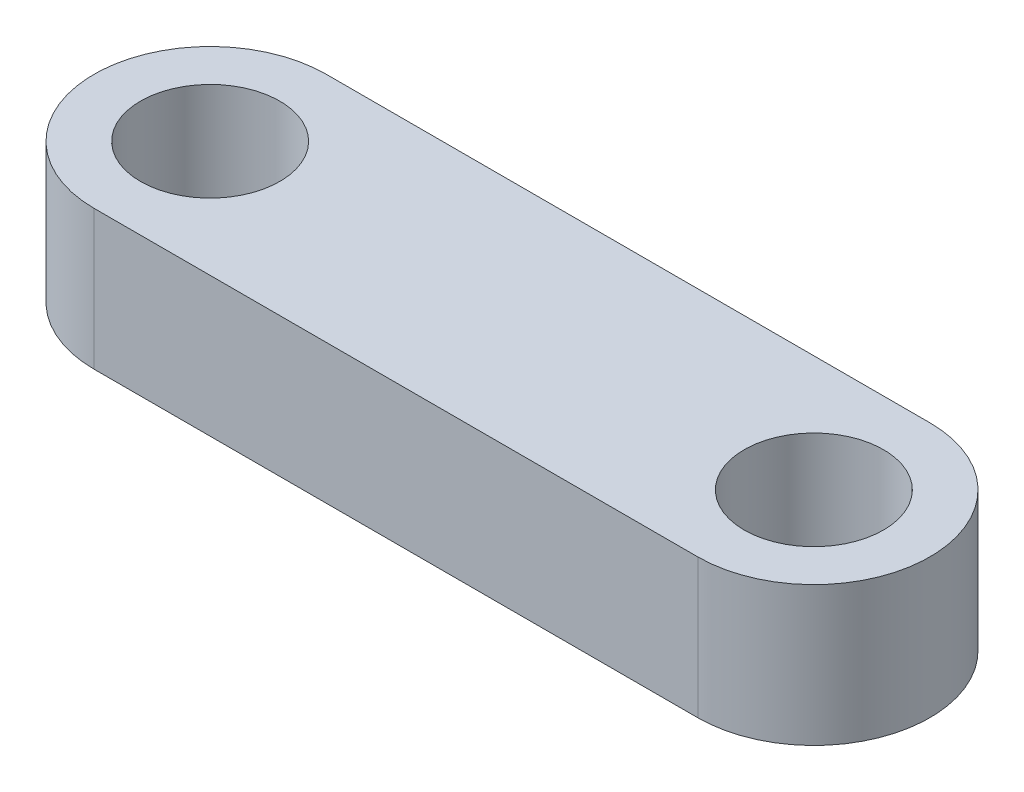
from build123d import *

# Parameters (mm, degrees)
SKETCH1_R           = 1.5
BOSS_EXTRUDE1_DEPTH = 3


with BuildPart() as part:
    # Sketch1 → Boss-Extrude1 (new body)
    with BuildSketch(Plane(origin=(0, 0, 0), x_dir=(1, 0, 0), z_dir=(0, 1, 0))):
        with BuildLine():
            Line((0, 2.5), (13, 2.5))
            ThreePointArc((13, 2.5), (15.5, 0), (13, -2.5))
            Line((13, -2.5), (0, -2.5))
            ThreePointArc((0, -2.5), (-2.5, 0), (0, 2.5))
        make_face()
        with Locations(Location((0, 0, 0), (0, 0, 270))):
            Circle(SKETCH1_R, mode=Mode.SUBTRACT)
        with Locations(Location((13, 0, 0), (0, 0, 270))):
            Circle(SKETCH1_R, mode=Mode.SUBTRACT)
    extrude(amount=BOSS_EXTRUDE1_DEPTH)


solid = part.part
